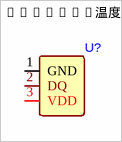
[diagram p0: symbol DS18B20温度传感器]
# Altium schematic symbol library MISC84237-13.SchLib: 1 symbol
Pins are listed as number, name and electrical type; pins without a type are passive.


## DS18B20温度传感器
designator U?
footprint DS18B20温度传感器 (Footprint not found)
pins: 1 GND, 2 DQ, 3 VDD